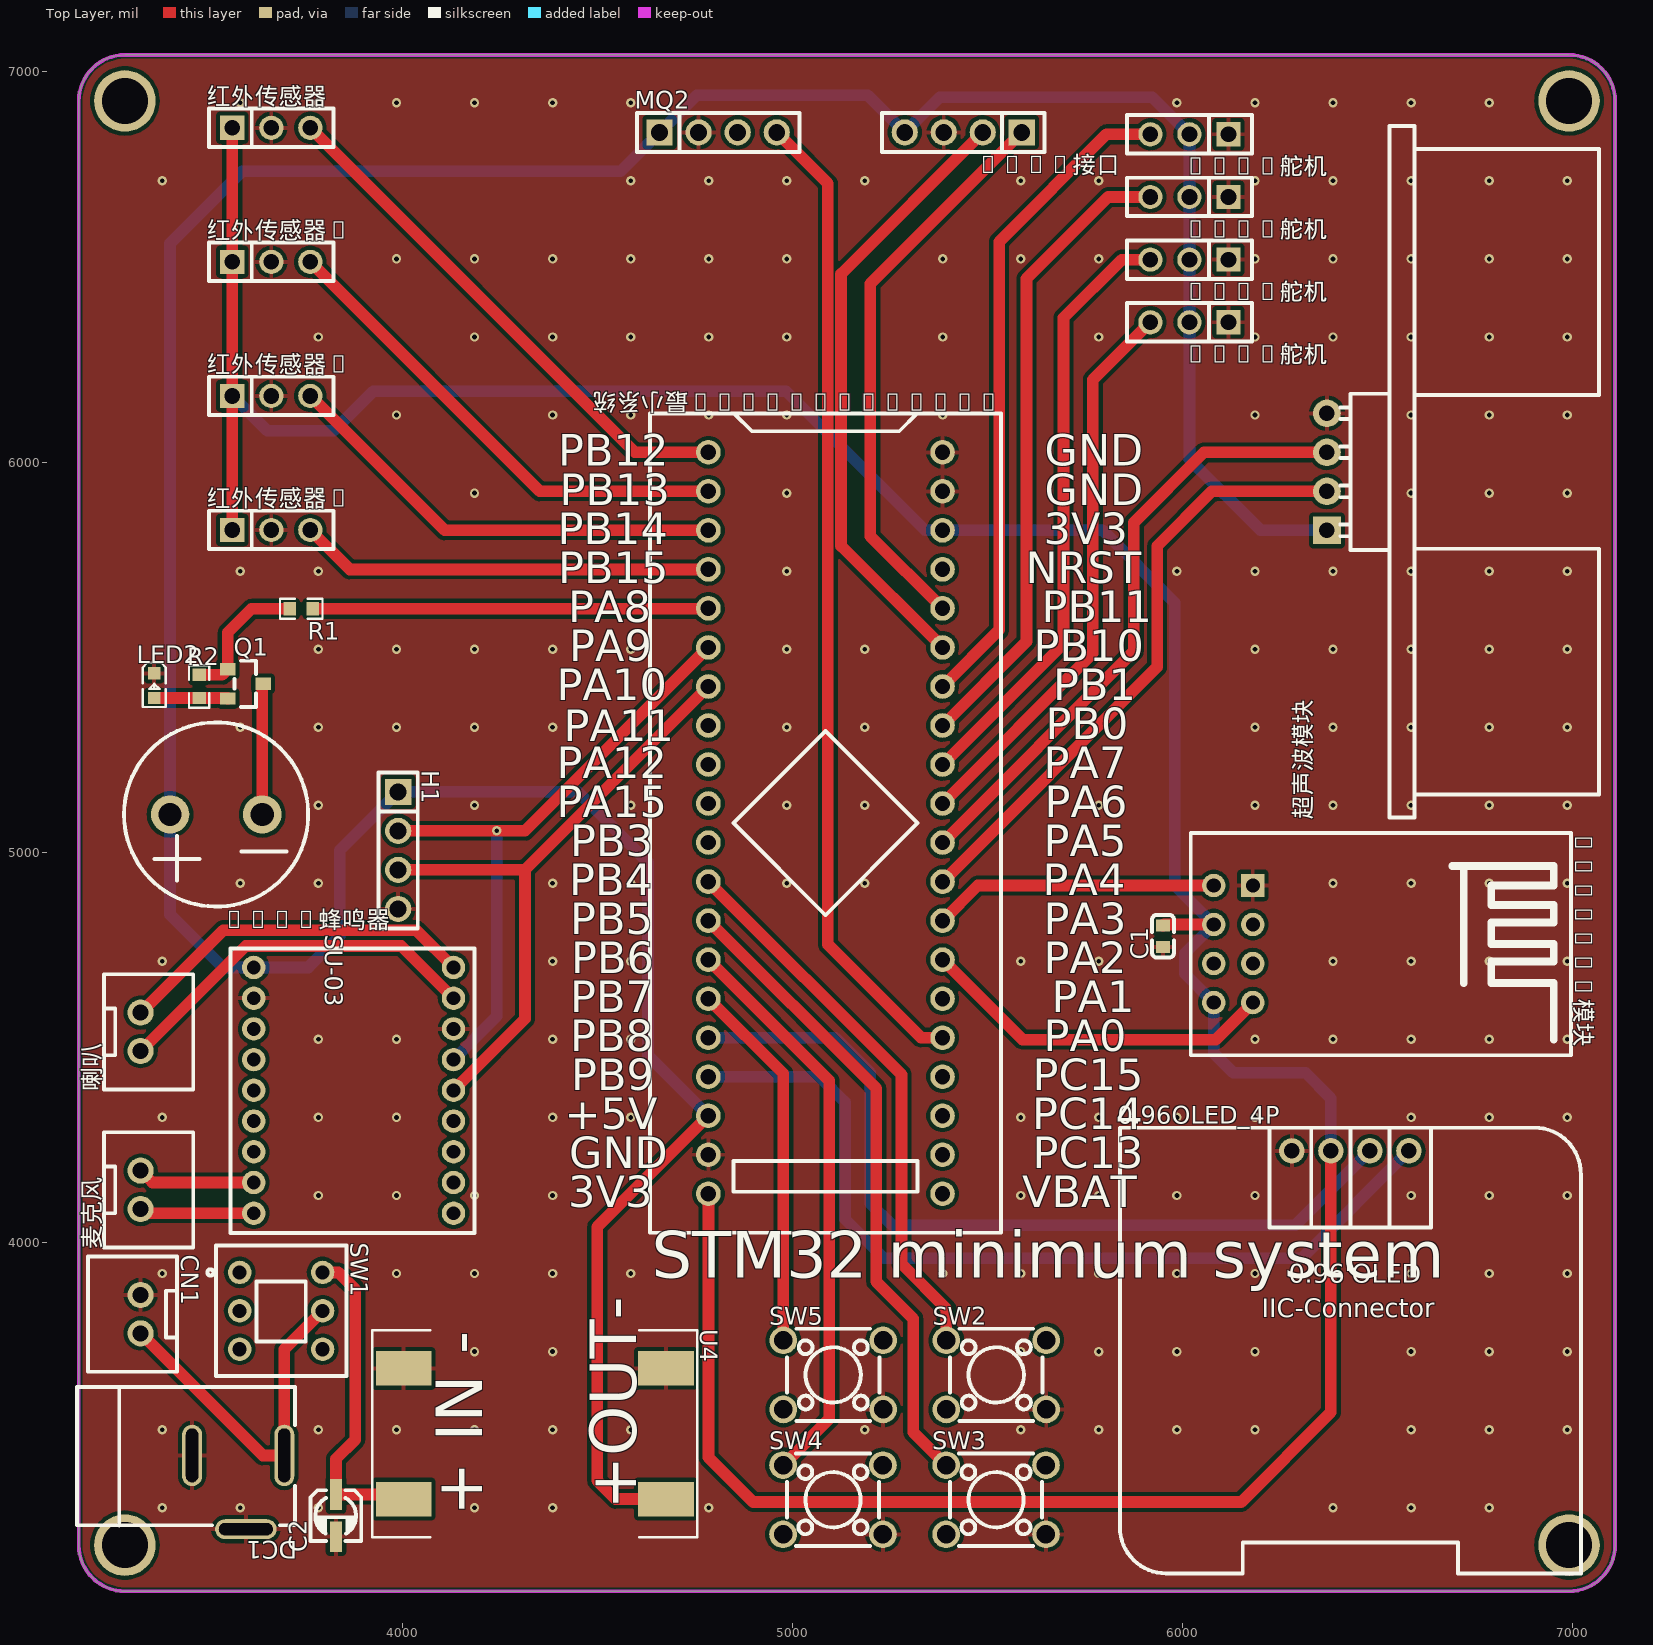
[diagram p0: Top Layer view]
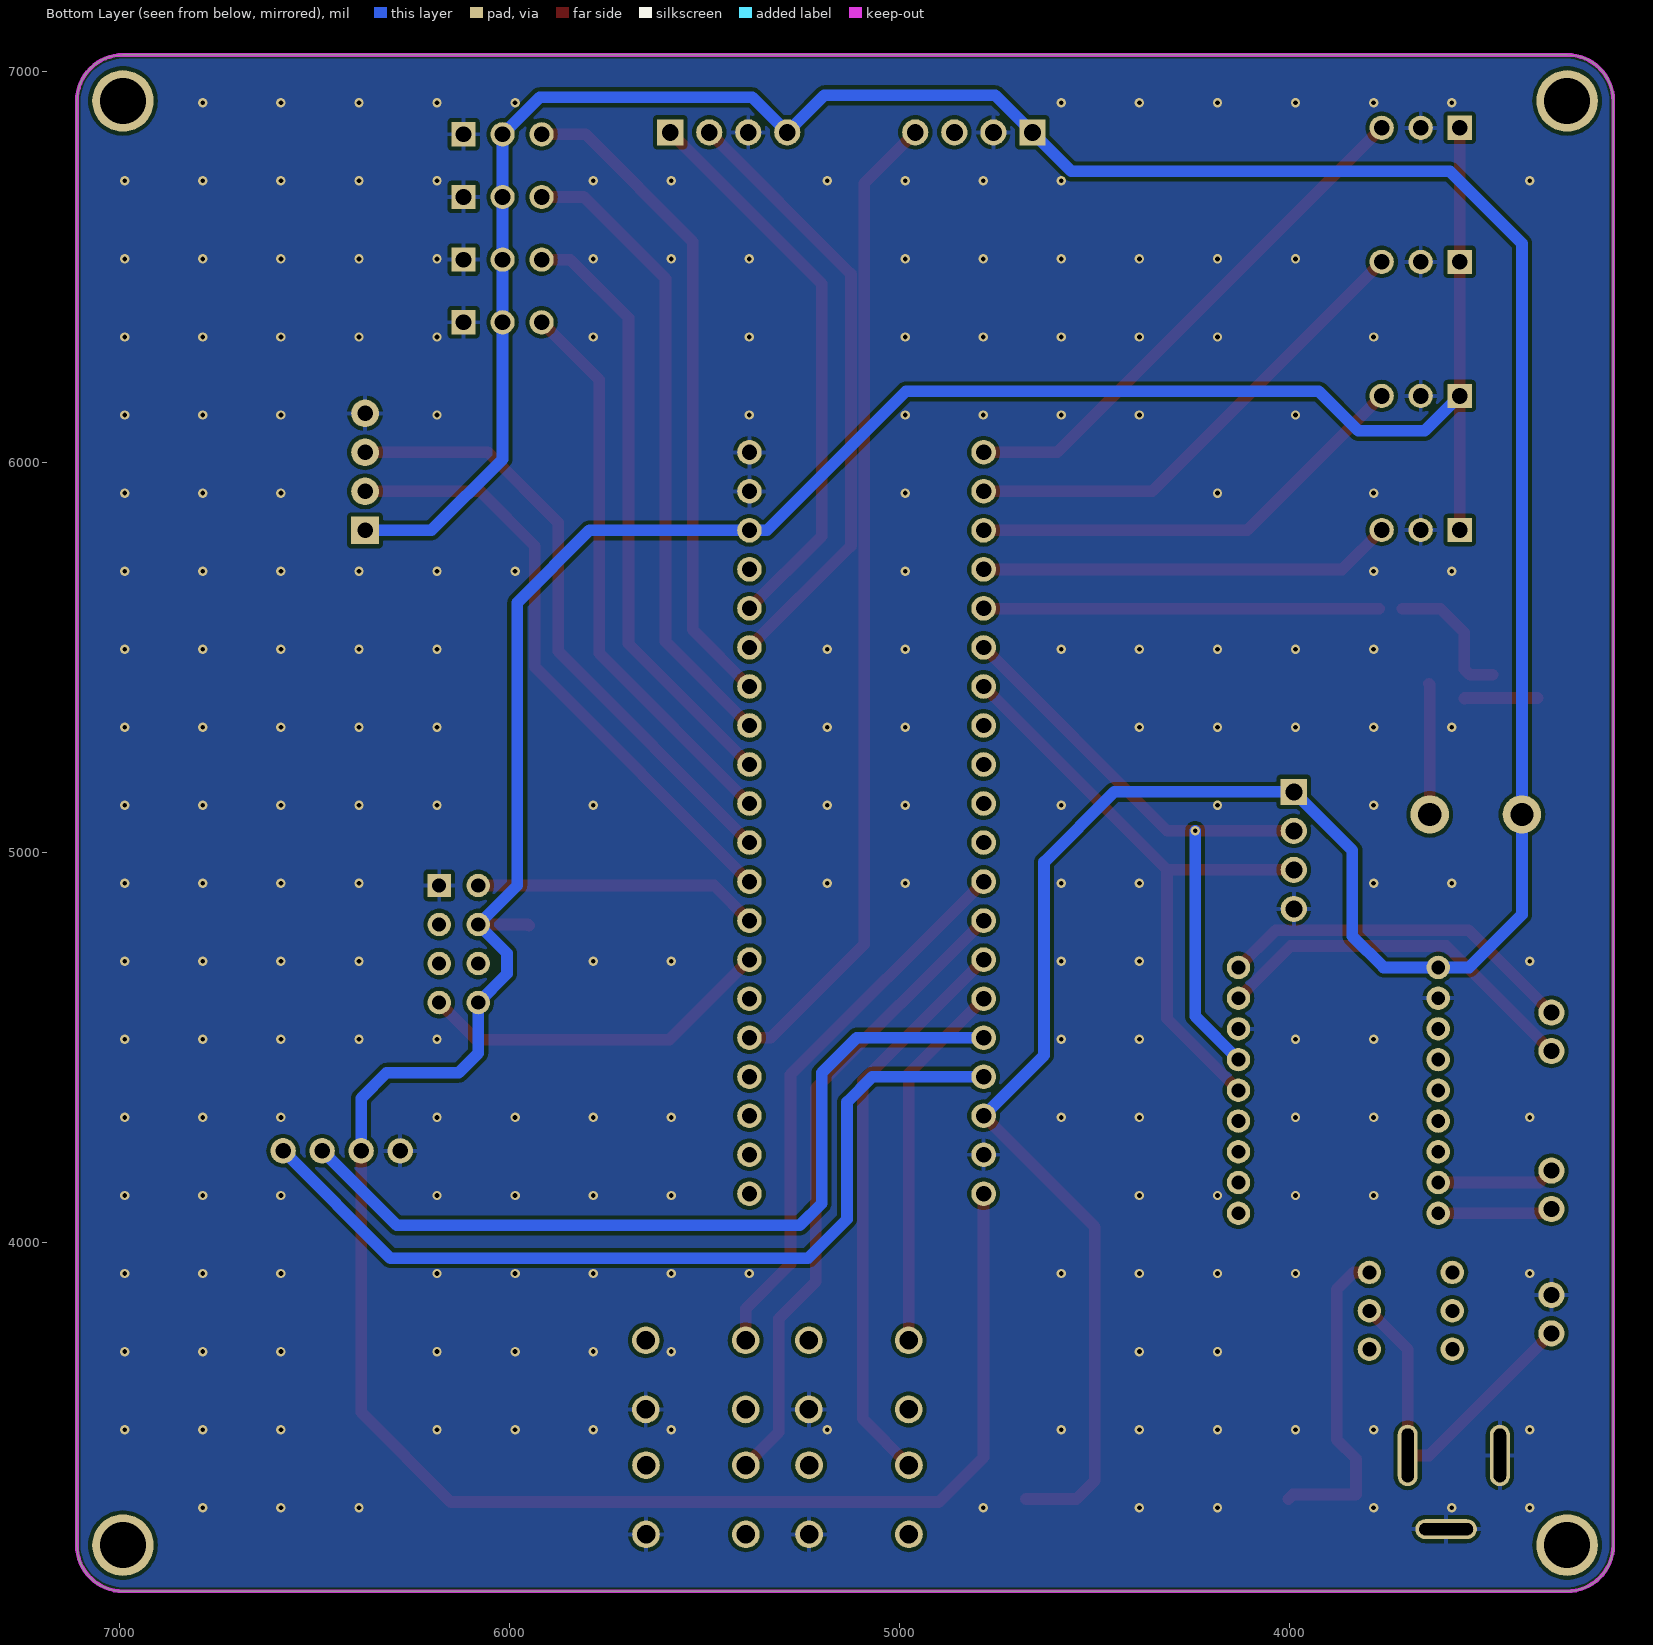
[diagram p1: Bottom Layer view, seen from below]
# Altium PCB MISC89030.pcbdoc
Units mil, origin at the board's own origin, x right, y up, seen from the top; angles counter-clockwise.
Board outline 3937.01 x 3937.01 mil, 2 copper layers (Top Layer, Bottom Layer), stack 62.206 mil thick; 33 components, 37 nets, 164 pads, 207 vias.

## Layer stack, top to bottom
Top Solder Mask Layer: solder mask 0.394, Dk 3.3
Top Layer: signal copper 1.379
Dielectric1: surface 59.449, FR4, Dk 4.5
Bottom Layer: signal copper 1.378
Bottom Solder Mask Layer: solder mask 0.394, Dk 3.3

## Board outline
6990.39,3106.5 ccw(c6990.39,3224.61) 7108.5,3224.61 7108.5,6925.39 ccw(c6990.39,6925.39) 6990.39,7043.5 3289.61,7043.5 ccw(c3289.61,6925.39) 3171.5,6925.39 3171.5,3224.61 ccw(c3289.61,3224.61) 3289.61,3106.5

## Design rules (kind name [scope] priority, off if disabled: settings)
BoardOutlineClearance copperThickness2oz_1 [All] p2 off: genericclearance=7.99 ignorepadtopadclearanceinfootprint=FALSE except(0: Arc-SplitContinuation Track-SplitContinuation SMDPad-SplitContinuation THPad-SplitContinuation Via-SplitContinuation Fill-SplitContinuation Region-SplitContinuation Poly-SplitContinuation Text-SplitContinuation Hole-SplitContinuation; 5.98: Arc-CutoutEdge Track-CutoutEdge SMDPad-CutoutEdge THPad-CutoutEdge Via-CutoutEdge Text-CutoutEdge; 6.89: Hole-OutlineEdge Hole-CutoutEdge; 10: Poly-OutlineEdge Poly-CutoutEdge; 11.81: Arc-OutlineEdge Track-OutlineEdge SMDPad-OutlineEdge THPad-OutlineEdge Via-OutlineEdge Fill-OutlineEdge Region-OutlineEdge Text-OutlineEdge Fill-CutoutEdge Region-CutoutEdge)
BoardOutlineClearance Plane_innerPlane_1 [All] p4 off: genericclearance=4.02 ignorepadtopadclearanceinfootprint=FALSE except(0: Arc-SplitContinuation Track-SplitContinuation SMDPad-SplitContinuation THPad-SplitContinuation Via-SplitContinuation Fill-SplitContinuation Region-SplitContinuation Poly-SplitContinuation Text-SplitContinuation Hole-SplitContinuation; 5.98: Arc-CutoutEdge Track-CutoutEdge SMDPad-CutoutEdge THPad-CutoutEdge Via-CutoutEdge Text-CutoutEdge; 6.89: Hole-OutlineEdge Hole-CutoutEdge; 10: Poly-OutlineEdge Poly-CutoutEdge; 11.81: Arc-OutlineEdge Track-OutlineEdge SMDPad-OutlineEdge THPad-OutlineEdge Via-OutlineEdge Fill-OutlineEdge Region-OutlineEdge Text-OutlineEdge Fill-CutoutEdge Region-CutoutEdge)
BoardOutlineClearance Copper_copperRegion_1 [All] p6 off: genericclearance=4.02 ignorepadtopadclearanceinfootprint=FALSE except(0: Arc-SplitContinuation Track-SplitContinuation SMDPad-SplitContinuation THPad-SplitContinuation Via-SplitContinuation Fill-SplitContinuation Region-SplitContinuation Poly-SplitContinuation Text-SplitContinuation Hole-SplitContinuation; 5.98: Arc-CutoutEdge Track-CutoutEdge SMDPad-CutoutEdge THPad-CutoutEdge Via-CutoutEdge Text-CutoutEdge; 6.89: Hole-OutlineEdge Hole-CutoutEdge; 10: Poly-OutlineEdge Poly-CutoutEdge; 11.81: Arc-OutlineEdge Track-OutlineEdge SMDPad-OutlineEdge THPad-OutlineEdge Via-OutlineEdge Fill-OutlineEdge Region-OutlineEdge Text-OutlineEdge Fill-CutoutEdge Region-CutoutEdge)
BoardOutlineClearance copperThickness1oz_1 [All] p8: genericclearance=4.02 ignorepadtopadclearanceinfootprint=FALSE except(0: Arc-SplitContinuation Track-SplitContinuation SMDPad-SplitContinuation THPad-SplitContinuation Via-SplitContinuation Fill-SplitContinuation Region-SplitContinuation Poly-SplitContinuation Text-SplitContinuation Hole-SplitContinuation; 5.98: Arc-CutoutEdge Track-CutoutEdge SMDPad-CutoutEdge THPad-CutoutEdge Via-CutoutEdge Text-CutoutEdge; 6.89: Hole-OutlineEdge Hole-CutoutEdge; 10: Poly-OutlineEdge Poly-CutoutEdge; 11.81: Arc-OutlineEdge Track-OutlineEdge SMDPad-OutlineEdge THPad-OutlineEdge Via-OutlineEdge Fill-OutlineEdge Region-OutlineEdge Text-OutlineEdge Fill-CutoutEdge Region-CutoutEdge)
Clearance copperThickness2oz [All] p1 off: gap=7.99 ignorepadtopadclearanceinfootprint=FALSE except(5.98: SMDPad-Track SMDPad-SMDPad THPad-Track SMDPad-THPad THPad-THPad Track-Via SMDPad-Via THPad-Via Via-Via Fill-SMDPad Region-SMDPad Fill-THPad Region-THPad Fill-Via Region-Via Fill-Fill Fill-Region Region-Region Arc-Track Arc-SMDPad Arc-THPad Arc-Via Fill-Arc Region-Arc Arc-Arc Text-Track SMDPad-Text Text-THPad Text-Via Fill-Text Region-Text Arc-Text Text-Text; 6.89: Hole-Track Hole-SMDPad Hole-THPad Hole-Via Fill-Hole Region-Hole Hole-Arc Hole-Text; 10: Poly-Track Poly-SMDPad Poly-THPad Poly-Via Poly-Fill Poly-Region Poly-Poly Poly-Arc Poly-Text Poly-Hole; 11.81: Fill-Track Region-Track)
Clearance Plane_innerPlane [All] p3 off: gap=4.02 ignorepadtopadclearanceinfootprint=FALSE except(5.98: SMDPad-Track SMDPad-SMDPad THPad-Track SMDPad-THPad THPad-THPad Track-Via SMDPad-Via THPad-Via Via-Via Fill-SMDPad Region-SMDPad Fill-THPad Region-THPad Fill-Via Region-Via Fill-Fill Fill-Region Region-Region Arc-Track Arc-SMDPad Arc-THPad Arc-Via Fill-Arc Region-Arc Arc-Arc Text-Track SMDPad-Text Text-THPad Text-Via Fill-Text Region-Text Arc-Text Text-Text; 6.89: Hole-Track Hole-SMDPad Hole-THPad Hole-Via Fill-Hole Region-Hole Hole-Arc Hole-Text; 10: Poly-Track Poly-SMDPad Poly-THPad Poly-Via Poly-Fill Poly-Region Poly-Poly Poly-Arc Poly-Text Poly-Hole; 11.81: Fill-Track Region-Track)
Clearance Copper_copperRegion [All] p5 off: gap=4.02 ignorepadtopadclearanceinfootprint=FALSE except(5.98: SMDPad-Track SMDPad-SMDPad THPad-Track SMDPad-THPad THPad-THPad Track-Via SMDPad-Via THPad-Via Via-Via Fill-SMDPad Region-SMDPad Fill-THPad Region-THPad Fill-Via Region-Via Fill-Fill Fill-Region Region-Region Arc-Track Arc-SMDPad Arc-THPad Arc-Via Fill-Arc Region-Arc Arc-Arc Text-Track SMDPad-Text Text-THPad Text-Via Fill-Text Region-Text Arc-Text Text-Text; 6.89: Hole-Track Hole-SMDPad Hole-THPad Hole-Via Fill-Hole Region-Hole Hole-Arc Hole-Text; 10: Poly-Track Poly-SMDPad Poly-THPad Poly-Via Poly-Fill Poly-Region Poly-Poly Poly-Arc Poly-Text Poly-Hole; 11.81: Fill-Track Region-Track)
Clearance copperThickness1oz [All] p7: gap=4.02 ignorepadtopadclearanceinfootprint=FALSE except(5.98: SMDPad-Track SMDPad-SMDPad THPad-Track SMDPad-THPad THPad-THPad Track-Via SMDPad-Via THPad-Via Via-Via Fill-SMDPad Region-SMDPad Fill-THPad Region-THPad Fill-Via Region-Via Fill-Fill Fill-Region Region-Region Arc-Track Arc-SMDPad Arc-THPad Arc-Via Fill-Arc Region-Arc Arc-Arc Text-Track SMDPad-Text Text-THPad Text-Via Fill-Text Region-Text Arc-Text Text-Text; 6.89: Hole-Track Hole-SMDPad Hole-THPad Hole-Via Fill-Hole Region-Hole Hole-Arc Hole-Text; 10: Poly-Track Poly-SMDPad Poly-THPad Poly-Via Poly-Fill Poly-Region Poly-Poly Poly-Arc Poly-Text Poly-Hole; 11.81: Fill-Track Region-Track)
DiffPairsRouting differentialPair [All] p1: maxlimit=6 minlimit=6 mostfreqgap=6 toplayer_minwidth=5 toplayer_prefwidth=10 toplayer_maxwidth=100 toplayer_mingap=6 toplayer_prefgap=6 toplayer_maxgap=6 bottomlayer_minwidth=5 bottomlayer_prefwidth=10 bottomlayer_maxwidth=100 bottomlayer_mingap=6 bottomlayer_prefgap=6 bottomlayer_maxgap=6 maxuncoupledlength=10
HoleToHoleClearance otherClearance [All] p1: gap=11.81 allowstackedmicrovias=TRUE
Length netLength [All] p1: minlimit=0 maxlimit=0
PasteMaskExpansion pasteMaskExpansion [All] p1: expansion=0
PlaneConnect innerPlane [All] p1: planeconnectstyle=Relief reliefexpansion=20 reliefentries=4 reliefconductorwidth=10 reliefairgap=10
PolygonConnect copperRegion [All] p1: connectstyle=Relief reliefconductorwidth=10 reliefentries=4 polygonreliefangle="90 Angle" airgapwidth=10 via.connectstyle=Relief via.reliefconductorwidth=10 via.reliefentries=4 via.polygonreliefangle="90 Angle" via.airgapwidth=10
RoutingVias viaSize [All] p1: holewidth=12.01 width=24.02 viastyle="Through Hole" minholewidth=11.81 minwidth=19.68 maxholewidth=248.03 maxwidth=393.7
SolderMaskExpansion solderMaskExpansion [IsVia] p1: expansion=-1000 istentingtop=TRUE
SolderMaskExpansion solderMaskExpansion [All] p2: expansion=2.01 istentingtop=FALSE
Width copperThickness2oz_2 [All] p1 off: maxlimit=100 minlimit=8 preferedwidth=10
Width copperThickness1oz_2 [All] p2: maxlimit=100 minlimit=5 preferedwidth=30

## Components (designator, comment, footprint, x,y, rotation, side; value= is the part's Value field where it differs from the comment)
0.96OLED_4P "" 0.96OLED_4P 6430,4235 r0 top
5VDC蜂鸣器 "buzzer" BUZ-TH_BD12.0-P6.00-D0.9-RD 3523.48,5097 r180 top
C1 "1uF" C0603 5950,4785 r90 top
C2 "1uF" C_Ele_SMD_3x5.4mm 3830,3300 r90 top
CN1 "XH2.54*2P_through-hole" CONN-TH_2P-P2.50-XH2.54-2P 3330,3816.57 r270 top
DC1 "" DC-2.0 3575,3465 r180 top
ESP-01S模块 "ESP8266-01S" WIFIM-TH_ESP8266-01S 6130,4765 r270 top
H1 "" HDR-TH_4P-P2.54-V-M 3990,5005 r270 top
K210接口 "" HDR-TH_4P-P2.54-V-F 5438.03,6845 r180 top
LED2 "" LED_0603 3365,5425 r270 top
MQ2 "" HDR-TH_4P-P2.54-V-F 4810,6845 r0 top
Q1 "" S8050_SOT-23 3598.48,5431.75 r180 top
R1 "1K" R0603 3741.65,5624.11 r180 top
R2 "10K" R0603 3480,5425 r90 top
SG90舵机 "" HDR-TH_3P-P2.54-V-F 6017.64,6358.27 r180 top
SG90舵机 "" HDR-TH_3P-P2.54-V-F 6017.64,6679.42 r180 top
SG90舵机 "" HDR-TH_3P-P2.54-V-F 6017.64,6518.85 r180 top
SG90舵机 "" HDR-TH_3P-P2.54-V-F 6017.64,6840 r180 top
STM32F103C8T6最小系统 "STM32F103C8T6-Card" CONN-TH_L53.3-W22.9_STM32F103C8T6-CARD 5085,5075 r270 top
SU-03 "CON2.0MM-PAD-18" CONN-TH_18P-P2.00_C9900078766 3620,4390 r270 top
SW1 "TK-6850-1" SW-TH_TK-6850-1 3690,3825 r270 top
SW2 "" SW-TH_4P-L6.0-W6.0-P4.50-LS6.5 5522.65,3660.85 r0 top
SW3 "" SW-TH_4P-L6.0-W6.0-P4.50-LS6.5 5522.03,3340.85 r0 top
SW4 "" SW-TH_4P-L6.0-W6.0-P4.50-LS6.5 5104.22,3340.85 r0 top
SW5 "" SW-TH_4P-L6.0-W6.0-P4.50-LS6.5 5104.84,3660.85 r0 top
U4 "" JYMK 4340,3510 r270 top
喇叭 "XH2.54*2P_through-hole" CONN-TH_2P-P2.50-XH2.54-2P 3330,4540 r90 top
红外传感器 "" HDR-TH_3P-P2.54-V-F 3664.74,6856.62 r0 top
红外传感器1 "" HDR-TH_3P-P2.54-V-F 3664.74,6513.07 r0 top
红外传感器2 "" HDR-TH_3P-P2.54-V-F 3664.74,6169.52 r0 top
红外传感器3 "" HDR-TH_3P-P2.54-V-F 3664.74,5825.98 r0 top
超声波模块 "HC-SR04" TH_HC-SR04V 6370,5975 r90 top
麦克风 "XH2.54*2P_through-hole" CONN-TH_2P-P2.50-XH2.54-2P 3330,4135 r90 top

## Footprints (in the part's own frame and the unit in brackets; to place one, negate y for a bottom-side part, rotate by r counter-clockwise, add the part's x,y. Pads: shape width x height; smd on the part's side, far side on the other; paste and mask are expansions set on the pad)
0.96OLED_4P [mm]
  round 1.65 hole 1 copper offset 0,0: 1(-3.81,-0.001) 2(-1.27,0.002) 3(1.27,0.002) 4(3.81,0.002)
  silkscreen extent -15,-27.5 15,1.5
BUZ-TH_BD12.0-P6.00-D0.9-RD [mm]
  round 2.5 hole 1.5 paste+0 mask+0.05: 1(-3,0) 2(3,0)
  silkscreen extent -5.99,-5.99 5.99,5.99
C0603 [mm]
  rect 0.8x0.9 smd: 1(-0.7,0) 2(0.7,0)
  silkscreen extent -1.39,-0.71 1.39,0.71
C_Ele_SMD_3x5.4mm [mil]
  rect 78.7x31.5 smd paste+0 mask+2: 1(54.1,-0.55) 2(-53.7,-0.55)
  silkscreen extent -65,-65 65,65
CONN-TH_2P-P2.50-XH2.54-2P [mm]
  round 1.7 hole 1.05 paste+0 mask+0.05: 1(1.25,0) 2(-1.25,0)
  silkscreen extent -3.75,-3.42 3.75,2.37
CONN-TH_18P-P2.00_C9900078766 [mil]
  round 60 hole 35.43 paste+0 mask+1.97: 1(-314.96,0.01) 2(-314.96,511.81) 3(-236.22,0.01) 4(-236.22,511.81) 5(-157.48,0.01) 6(-157.48,511.81) 9(0,0) 10(0,511.81) 11(78.74,0) 12(78.74,511.81) 13(157.48,0) 14(157.48,511.81) 15(236.22,0) 16(236.22,511.81) 17(314.96,0) 18(314.96,511.81)
  round 60 hole 35.43 copper offset -0.01,0 paste+0 mask+1.97: 7(-78.72,0.01) 8(-78.72,511.81)
  silkscreen extent -363,-60 365,565
CONN-TH_L53.3-W22.9_STM32F103C8T6-CARD [mm]
  round 1.6 hole 1: 1(-24.13,-7.62) 2(-21.59,-7.62) 3(-19.05,-7.62) 4(-16.51,-7.62) 5(-13.97,-7.62) 6(-11.43,-7.62) 7(-8.89,-7.62) 8(-6.35,-7.62) 9(-3.81,-7.62) 10(-1.27,-7.62) 11(1.27,-7.62) 12(3.81,-7.62) 13(6.35,-7.62) 14(8.89,-7.62) 15(11.43,-7.62) 16(13.97,-7.62) 17(16.51,-7.62) 18(19.05,-7.62) 19(21.59,-7.62) 20(24.13,-7.62) 21(24.13,7.62) 22(21.59,7.62) 23(19.05,7.62) 24(16.51,7.62) 25(13.97,7.62) 26(11.43,7.62) 27(8.89,7.62) 28(6.35,7.62) 29(3.81,7.62) 30(1.27,7.62) 31(-1.27,7.62) 32(-3.81,7.62) 33(-6.35,7.62) 34(-8.89,7.62) 35(-11.43,7.62) 36(-13.97,7.62) 37(-16.51,7.62) 38(-19.05,7.62) 39(-21.59,7.62) 40(-24.13,7.62)
  silkscreen extent -26.67,-11.43 26.67,11.43
DC-2.0 [mil]
  oval 157.5x51.2 hole 31.5 slot 137.8 at 0 deg paste+0 mask+2: 2(-24.7,199.5)
  oval 51.2x157.5 hole 31.5 slot 137.8 at 90 deg paste+0 mask+2: 3(113.1,10.5) 4(-123.1,10.5)
  silkscreen extent -151,-165 408,190
HDR-TH_3P-P2.54-V-F [mil]
  rect 62x62 hole 40.16: 1(-100,0)
  round 62 hole 40.16: 2(0,0) 3(100,0)
  silkscreen extent -160,-49 160,49
HDR-TH_4P-P2.54-V-F [mm]
  rect 1.7x1.7 hole 1.1: 1(-3.81,0)
  round 1.7 hole 1.1: 2(-1.27,0) 3(1.27,0) 4(3.81,0)
  silkscreen extent -5.29,-1.27 5.29,1.27
HDR-TH_4P-P2.54-V-M [mm]
  rect 1.7x1.7 hole 1.1: 1(-3.81,0)
  round 1.7 hole 1.1: 2(-1.27,0) 3(1.27,0) 4(3.81,0)
  silkscreen extent -5.08,-1.27 5.08,1.27
JYMK [mm]
  rect 2.25x3.625 smd: 1(-4.25,-8.537) 2(4.25,-8.537) 3(4.25,8.537) 4(-4.25,8.537)
  silkscreen extent -6.73,-10.58 6.73,10.58
LED_0603 [mil]
  rect 31.5x31.5 smd paste+0 mask+2: 1(-33.5,-0.4) 2(29.5,-0.2)
  silkscreen extent -61,-30 53,30
R0603 [mil]
  rect 31.75x34.02 smd paste-3937.01 mask+2: 1(-29.66,0) 2(29.66,0)
  silkscreen extent -55,-26 55,26
S8050_SOT-23 [mm]
  rect 1x0.8 smd paste+0 mask+0.051: 1(1.15,-0.95) 2(1.15,0.95) 3(-1.15,0)
  silkscreen extent -0.7,-1.5 0.7,1.5
SW-TH_4P-L6.0-W6.0-P4.50-LS6.5 [mm]
  round 1.8 hole 1.2: 1(-3.25,2.25) 2(3.25,2.25) 3(-3.25,-2.25) 4(3.25,-2.25)
  silkscreen extent -3,-3 3,3
SW-TH_TK-6850-1 [mil]
  round 60 hole 35.98: 1(-98.43,-106.3) 2(-0.01,-106.3) 3(98.42,-106.3)
  round 60 hole 36: 4(-98.43,106.3) 5(-0.01,106.3) 6(98.42,106.3)
  silkscreen extent -167,-189 167,167
TH_HC-SR04V [mm]
  rect 1.8x1.8 hole 1.001: 1(-3.81,0)
  round 1.8 hole 1.001: 2(-1.27,0) 3(1.27,0) 4(3.81,0)
  silkscreen extent -22.5,-17.7 22.5,-0.89
WIFIM-TH_ESP8266-01S [mil]
  rect 60x60 hole 36 paste+0 mask+1.97: 1(-150,50)
  round 60 hole 36 paste+0 mask+1.97: 2(-50,50) 3(50,50) 4(150,50) 5(-150,-50) 6(-50,-50) 7(50,-50) 8(150,-50)
  silkscreen extent -285,-109 285,866

## Free pads (board coordinates)
  round 157.48 hole 118.11: 1(3289.61,6925.39) 1(3289.61,3224.61) 1(6990.39,6925.39) 1(6990.39,3224.61)

## Via types
v1: diameter 24.02, hole 12, Top Layer to Bottom Layer, 207 vias

## Nets (pads, with @x,y where several pads share a name; then routed paths per layer and width w, separated by ;. In a path a pad name is that pad's centre, name@x,y a point inside that pad or via, vN(x,y) a via of type N, cw(c..) or ccw(c..) an arc to the next point about the centre after c; other vN are vias at no path point)
$1N18192: Q1.1 R1.2 R2.2 | length 357.3
  Top Layer w30: R2.2 3538.71,5454.66 Q1.1 3553.2,5563.2 3614.11,5624.11 R1.2
$1N18194: LED2.2 Q1.2 R2.1 | length 188.9
  Top Layer w30: LED2.2 3552.05,5395.5 Q1.2
$1N18196: 5VDC蜂鸣器.1 Q1.3 | length 335.6
  Top Layer w30: 5VDC蜂鸣器.1 3641.59,5429.58 Q1.3
$1N18242: C2.1 SW1.4 U4.2 | length 826.1
  Top Layer w30: SW1.4 3836.57,3923.43 3880,3880 3880,3495 3830.55,3445.55 C2.1 3992.46,3354.1 U4.2
+5V: 5VDC蜂鸣器.2 H1.1 K210接口.4 MQ2.1 SG90舵机.2 STM32F103C8T6最小系统.18 SU-03.1 U4.3 超声波模块.1 | length 9500
  Top Layer w30: U4.3 4547.32,3342.68 4500,3390 4500,4040 STM32F103C8T6最小系统.18
  Bottom Layer w30: STM32F103C8T6最小系统.18 4630,4480 4630,4975 4450,5155 H1.1 3840,5005 3840,4785 3759.96,4704.96 SU-03.1 3540.04,4704.96 3405.37,4839.63 5VDC蜂鸣器.2 3405.37,6560.37 3590,6745 4560,6745 MQ2.1 4755,6940 5193.03,6940 K210接口.4 5378.03,6935 5922.64,6935 6017.64,6840 6017.64,6679.42 6017.64,6518.85 6017.64,6358.27 6017.64,6007.36 6200,5825 超声波模块.1
+7.8V: CN1.1 DC1.4 SW1.5 | length 908.9
  Top Layer w30: CN1.1 3642.86,3454.5 DC1.4 3698.1,3726.8 SW1.5
GND: 0.96OLED_4P.1 C1.1 C2.2 CN1.2 DC1.2 DC1.3 ESP-01S模块.1 H1.4 K210接口.3 LED2.1 MQ2.2 SG90舵机.1 STM32F103C8T6最小系统.19 STM32F103C8T6最小系统.39 STM32F103C8T6最小系统.40 SU-03.3 SU-03.6 SW2.4 SW3.4 SW4.4 SW5.4 U4.1 U4.4 红外传感器1.2 红外传感器2.2 红外传感器3.2 红外传感器.2 超声波模块.4
  other v1: 3385.6,3320.6 3585.6,3320.6 3785.6,3320.6 4185.6,3320.6 4385.6,3320.6 4785.6,3320.6 6385.6,3320.6 6585.6,3320.6 6785.6,3320.6 3385.6,3520.6 3785.6,3520.6 3985.6,3520.6 4185.6,3520.6 4385.6,3520.6 4585.6,3520.6 5185.6,3520.6 5585.6,3520.6 5785.6,3520.6 5985.6,3520.6 6185.6,3520.6 6585.6,3520.6 6785.6,3520.6 6985.6,3520.6 4185.6,3720.6 4385.6,3720.6 5585.6,3720.6 5785.6,3720.6 5985.6,3720.6 6185.6,3720.6 6585.6,3720.6 6785.6,3720.6 6985.6,3720.6 3385.6,3920.6 3985.6,3920.6 4185.6,3920.6 4385.6,3920.6 4585.6,3920.6 5385.6,3920.6 5585.6,3920.6 5785.6,3920.6 5985.6,3920.6 6185.6,3920.6 6585.6,3920.6 6785.6,3920.6 6985.6,3920.6 3785.6,4120.6 3985.6,4120.6 4185.6,4120.6 4385.6,4120.6 5585.6,4120.6 5785.6,4120.6 5985.6,4120.6 6185.6,4120.6 6585.6,4120.6 6785.6,4120.6 6985.6,4120.6 3385.6,4320.6 3785.6,4320.6 3985.6,4320.6 4385.6,4320.6 4585.6,4320.6 5585.6,4320.6 5785.6,4320.6 5985.6,4320.6 6185.6,4320.6 6585.6,4320.6 6785.6,4320.6 6985.6,4320.6 3785.6,4520.6 3985.6,4520.6 4385.6,4520.6 4585.6,4520.6 6185.6,4520.6 6385.6,4520.6 6585.6,4520.6 6785.6,4520.6 6985.6,4520.6 3385.6,4720.6 4385.6,4720.6 4585.6,4720.6 5585.6,4720.6 5785.6,4720.6 6385.6,4720.6 6585.6,4720.6 6785.6,4720.6 6985.6,4720.6 3585.6,4920.6 3785.6,4920.6 4385.6,4920.6 4585.6,4920.6 4985.6,4920.6 5185.6,4920.6 6385.6,4920.6 6585.6,4920.6 6785.6,4920.6 6985.6,4920.6 3785.6,5120.6 4185.6,5120.6 4585.6,5120.6 4985.6,5120.6 5185.6,5120.6 5785.6,5120.6 6185.6,5120.6 6385.6,5120.6 6585.6,5120.6 6785.6,5120.6 6985.6,5120.6 3585.6,5320.6 3785.6,5320.6 3985.6,5320.6 4185.6,5320.6 4385.6,5320.6 4985.6,5320.6 5185.6,5320.6 6185.6,5320.6 6385.6,5320.6 6585.6,5320.6 6785.6,5320.6 6985.6,5320.6 3785.6,5520.6 3985.6,5520.6 4185.6,5520.6 4385.6,5520.6 4585.6,5520.6 4985.6,5520.6 5185.6,5520.6 6185.6,5520.6 6385.6,5520.6 6585.6,5520.6 6785.6,5520.6 6985.6,5520.6 3585.6,5720.6 3785.6,5720.6 4985.6,5720.6 5985.6,5720.6 6185.6,5720.6 6385.6,5720.6 6585.6,5720.6 6785.6,5720.6 6985.6,5720.6 3785.6,5920.6 4185.6,5920.6 4985.6,5920.6 6585.6,5920.6 6785.6,5920.6 6985.6,5920.6 3985.6,6120.6 4385.6,6120.6 4585.6,6120.6 4785.6,6120.6 4985.6,6120.6 5385.6,6120.6 6185.6,6120.6 6585.6,6120.6 6785.6,6120.6 6985.6,6120.6 3785.6,6320.6 4185.6,6320.6 4385.6,6320.6 4585.6,6320.6 4785.6,6320.6 4985.6,6320.6 5385.6,6320.6 5785.6,6320.6 6185.6,6320.6 6385.6,6320.6 6585.6,6320.6 6785.6,6320.6 6985.6,6320.6 3985.6,6520.6 4185.6,6520.6 4385.6,6520.6 4585.6,6520.6 4785.6,6520.6 4985.6,6520.6 5385.6,6520.6 5585.6,6520.6 5785.6,6520.6 6185.6,6520.6 6385.6,6520.6 6585.6,6520.6 6785.6,6520.6 6985.6,6520.6 3385.6,6720.6 4585.6,6720.6 4785.6,6720.6 4985.6,6720.6 5185.6,6720.6 5585.6,6720.6 5785.6,6720.6 6185.6,6720.6 6385.6,6720.6 6585.6,6720.6 6785.6,6720.6 6985.6,6720.6 3585.6,6920.6 3785.6,6920.6 3985.6,6920.6 4185.6,6920.6 4385.6,6920.6 4585.6,6920.6 5985.6,6920.6 6185.6,6920.6 6385.6,6920.6 6585.6,6920.6 6785.6,6920.6
MIC+: SU-03.15 麦克风.1 | length 302.6
  Top Layer w30: 麦克风.1 3360.43,4153.78 SU-03.15
MIC-: SU-03.17 麦克风.2 | length 294.5
  Top Layer w30: 麦克风.2 3340.74,4075.04 SU-03.17
PA0: MQ2.4 STM32F103C8T6最小系统.25 | length 2528.3
  Top Layer w30: MQ2.4 5090.98,6714.02 5090.98,4764.02 5330,4525 STM32F103C8T6最小系统.25
PA1: STM32F103C8T6最小系统.26
PA2: ESP-01S模块.4 STM32F103C8T6最小系统.27 | length 919.3
  Top Layer w30: STM32F103C8T6最小系统.27 5590,4520 6085,4520 ESP-01S模块.4
PA3: ESP-01S模块.5 STM32F103C8T6最小系统.28 | length 732.3
  Top Layer w30: STM32F103C8T6最小系统.28 5475,4915 ESP-01S模块.5
PA4: STM32F103C8T6最小系统.29 超声波模块.2 | length 1580.8
  Top Layer w30: STM32F103C8T6最小系统.29 5935,5475 5935,5785 6075,5925 超声波模块.2
PA5: STM32F103C8T6最小系统.30 超声波模块.3 | length 1592.5
  Top Layer w30: STM32F103C8T6最小系统.30 5875,5515 5875,5845 6055,6025 超声波模块.3
PA6: SG90舵机.3@5917.64,6358.27 STM32F103C8T6最小系统.31 | length 1453.9
  Top Layer w30: STM32F103C8T6最小系统.31 5770,5510 5770,6210.63 SG90舵机.3@5917.64,6358.27
PA7: SG90舵机.3@5917.64,6518.85 STM32F103C8T6最小系统.32 | length 1557.7
  Top Layer w30: STM32F103C8T6最小系统.32 5695,5535 5695,6370 5843.85,6518.85 SG90舵机.3@5917.64,6518.85
PA8: R1.1 STM32F103C8T6最小系统.5 | length 1014.1
  Top Layer w30: R1.1 4784.11,5624.11 STM32F103C8T6最小系统.5
PA9: H1.2 STM32F103C8T6最小系统.6 SU-03.8 | length 1621.9
  Top Layer w30: H1.2 v1(4242.83,5055) 4315,5055 STM32F103C8T6最小系统.6
  Bottom Layer w30: SU-03.8 4242.83,4579.74 v1(4242.83,5055)
PA10: H1.3 STM32F103C8T6最小系统.7 SU-03.10 | length 1630.6
  Top Layer w30: H1.3 4315,4955 ; SU-03.10 4315,4573.19 4315,4955 ; STM32F103C8T6最小系统.7 4315,4955
PB0: SG90舵机.3@5917.64,6679.42 STM32F103C8T6最小系统.33 | length 1638.4
  Top Layer w30: STM32F103C8T6最小系统.33 5600,5540 5600,6470 5809.42,6679.42 SG90舵机.3@5917.64,6679.42
PB1: SG90舵机.3@5917.64,6840 STM32F103C8T6最小系统.34 | length 1701.6
  Top Layer w30: STM32F103C8T6最小系统.34 5530,5570 5530,6565 5805,6840 SG90舵机.3@5917.64,6840
PB4: STM32F103C8T6最小系统.12 SW2.1 | length 1428.1
  Top Layer w30: STM32F103C8T6最小系统.12 5280,4430 5280,3945 5394.7,3830.3 SW2.1
PB5: STM32F103C8T6最小系统.13 SW3.1 | length 1647.9
  Top Layer w30: STM32F103C8T6最小系统.13 5215,4395 5215,3900 5310,3805 5310,3513.51 SW3.1
PB6: STM32F103C8T6最小系统.14 SW4.1 | length 1473.2
  Top Layer w30: STM32F103C8T6最小系统.14 5095,4415 5095,3548.16 SW4.1
PB7: STM32F103C8T6最小系统.15 SW5.1 | length 955.1
  Top Layer w30: STM32F103C8T6最小系统.15 4976.89,4433.11 SW5.1
PB8: 0.96OLED_4P.3 STM32F103C8T6最小系统.16 | length 2169.6
  Bottom Layer w30: STM32F103C8T6最小系统.16 5110,4525 5200,4435 5200,4100 5255.98,4044.02 6288.97,4044.02 0.96OLED_4P.3@6480,4235.05
PB9: 0.96OLED_4P.4 STM32F103C8T6最小系统.17 | length 2277.3
  Bottom Layer w30: STM32F103C8T6最小系统.17 5070,4425 5135,4360 5135,4060 5235,3960 6304.95,3960 0.96OLED_4P.4@6580,4235.05
PB10: K210接口.2 STM32F103C8T6最小系统.35 | length 1578.1
  Top Layer w30: STM32F103C8T6最小系统.35 5125,5785 5125,6481.97 K210接口.2
PB11: K210接口.1 STM32F103C8T6最小系统.36 | length 1457.4
  Top Layer w30: STM32F103C8T6最小系统.36 5200,5810 5200,6456.97 K210接口.1
PB12: STM32F103C8T6最小系统.1 红外传感器.3 | length 1364.7
  Top Layer w30: 红外传感器.3 4596.36,6025 STM32F103C8T6最小系统.1
PB13: STM32F103C8T6最小系统.2 红外传感器1.3 | length 1263.8
  Top Layer w30: 红外传感器1.3 4352.81,5925 STM32F103C8T6最小系统.2
PB14: STM32F103C8T6最小系统.3 红外传感器2.3 | length 1163
  Top Layer w30: 红外传感器2.3 4109.27,5825 STM32F103C8T6最小系统.3
PB15: STM32F103C8T6最小系统.4 红外传感器3.3 | length 1062.1
  Top Layer w30: 红外传感器3.3 3865.72,5725 STM32F103C8T6最小系统.4
SPK+: SU-03.2 喇叭.1 | length 928.9
  Top Layer w30: 喇叭.1 3541.34,4800.55 4036.22,4800.55 SU-03.2
SPK-: SU-03.4 喇叭.2 | length 968.7
  Top Layer w30: 喇叭.2 3599.22,4760 3998.03,4760 SU-03.4
VCC: 0.96OLED_4P.2 C1.2 ESP-01S模块.6 ESP-01S模块.8 STM32F103C8T6最小系统.20 STM32F103C8T6最小系统.38 红外传感器1.1 红外传感器2.1 红外传感器3.1 红外传感器.1 | length 8703.2
  Top Layer w30: 红外传感器3.1 红外传感器2.1 红外传感器1.1 红外传感器.1 ; STM32F103C8T6最小系统.20 4785,3450 4900,3335 6150,3335 6380,3565 0.96OLED_4P.2@6380,4235.05 ; C1.2 5952.44,4815 ESP-01S模块.6
  Bottom Layer w30: 红外传感器2.1 3654.26,6080 3825,6080 3926.21,6181.21 4983.79,6181.21 5340,5825 STM32F103C8T6最小系统.38 5795,5825 5980,5640 5980,4915 ESP-01S模块.6 6006.21,4741.21 6006.21,4688.79 ESP-01S模块.8 6080,4485 6130,4435 6315,4435 6380,4370 0.96OLED_4P.2@6380,4235.05
pads on no net: ESP-01S模块.2 ESP-01S模块.3 ESP-01S模块.7 MQ2.3 STM32F103C8T6最小系统.8 STM32F103C8T6最小系统.9 STM32F103C8T6最小系统.10 STM32F103C8T6最小系统.11 STM32F103C8T6最小系统.21 STM32F103C8T6最小系统.22 STM32F103C8T6最小系统.23 STM32F103C8T6最小系统.24 STM32F103C8T6最小系统.37 SU-03.5 SU-03.7 SU-03.9 SU-03.11 SU-03.12 SU-03.13 SU-03.14 SU-03.16 SU-03.18 SW1.1 SW1.2 SW1.3 SW1.6 SW2.2 SW2.3 SW3.2 SW3.3 SW4.2 SW4.3 SW5.2 SW5.3

## Polygon pours and split planes (outlines as drawn)
GND on Bottom Layer (solid, remove dead copper, pour order 2): 3100,7165 3100,3000 7275,3000 7275,7165
GND on Top Layer (solid, remove dead copper, pour order 0): 3000,7145 3000,3075 7385,3075 7385,7145

## Keep-outs
Board Outline Layer:
  the board outline again, w10

## Silkscreen, mask and mechanical layers (free items; w line width, h text height)
Top Silkscreen Layer:
  text "PB12" at 4400.64,5990 h80
  text "GND" at 5646.65,5990 h80
  text "PB13" at 4403.85,5890 h80
  text "GND" at 5646.65,5890 h80
  text "PB14" at 4398.34,5790 h80
  text "3V3" at 5644.45,5790 h80
  text "PB15" at 4400.64,5690 h80
  text "NRST" at 5598.65,5690 h80
  text "PA8" at 4426.24,5590 h80
  text "PB11" at 5639.05,5590 h80
  text "PA9" at 4428.44,5490 h80
  text "PB10" at 5618.85,5490 h80
  text "PA10" at 4396.14,5390 h80
  text "PB1" at 5669.15,5390 h80
  text "PB0" at 5648.95,5290 h80
  text "PA11" at 4414.55,5285 h80
  text "PA12" at 4396.14,5190 h80
  text "PA7" at 5644.45,5190 h80
  text "PA15" at 4396.14,5090 h80
  text "PA6" at 5646.65,5090 h80
  text "PB3" at 4430.74,4990 h80
  text "PA5" at 5644.45,4990 h80
  text "PB4" at 4428.44,4890 h80
  text "PA4" at 5642.15,4890 h80
  text "PB5" at 4430.74,4790 h80
  text "PA3" at 5644.45,4790 h80
  text "PB6" at 4432.94,4690 h80
  text "PA2" at 5644.45,4690 h80
  text "PB7" at 4430.74,4590 h80
  text "PA1" at 5664.65,4590 h80
  text "PB8" at 4430.74,4490 h80
  text "PA0" at 5644.45,4490 h80
  text "PB9" at 4432.94,4390 h80
  text "PC15" at 5616.55,4390 h80
  text "+5V" at 4417.24,4290 h80
  text "PC14" at 5614.25,4290 h80
  text "GND" at 4428.44,4190 h80
  text "PC13" at 5616.55,4190 h80
  text "3V3" at 4426.24,4090 h80
  text "VBAT" at 5589.65,4090 h80
  text "STM32 minimum system" at 4640,3910 h120